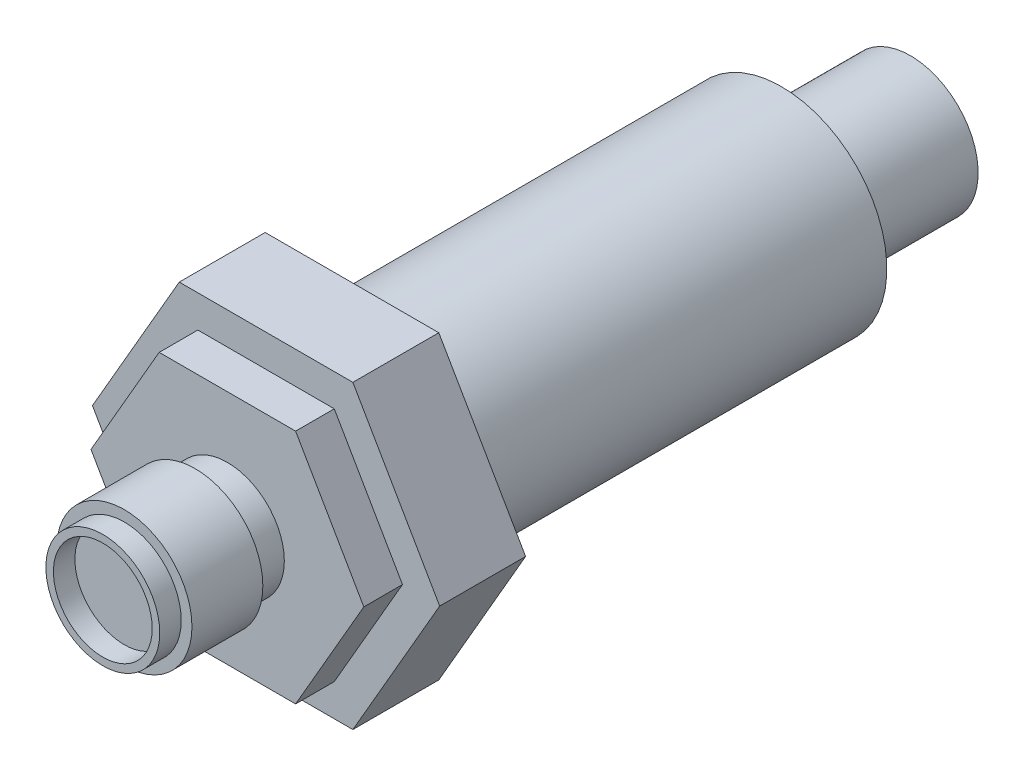
SolidWorks part; units mm, degrees
ref_plane "Front Plane" through (0, 0, 0) normal (0, 0, 1) x (1, 0, 0)
ref_plane "Top Plane" through (0, 0, 0) normal (0, 1, 0) x (1, 0, 0)
ref_plane "Right Plane" through (0, 0, 0) normal (1, 0, 0) x (0, 0, -1)
sketch "Sketch1" plane through (0, 0, 0) normal (0, 0, 1) x (1, 0, 0)
  line L1 (8.0829, 0) -> (4.0415, 7)
  line L2 (4.0415, 7) -> (-4.0415, 7)
  line L3 (-4.0415, 7) -> (-8.0829, 0)
  line L4 (-8.0829, 0) -> (-4.0415, -7)
  line L5 (-4.0415, -7) -> (4.0415, -7)
  line L6 (4.0415, -7) -> (8.0829, 0)
  circle A0 centre (0, 0) radius 7 construction
  dimension "D1" = 14
extrude "Boss-Extrude1" add sketch "Sketch1" along normal blind 4
sketch "Sketch2" plane through (0, 0, 4) normal (0, 0, 1) x (1, 0, 0)
  line L1 (6.3509, 0) -> (3.1754, 5.5)
  line L2 (3.1754, 5.5) -> (-3.1754, 5.5)
  line L3 (-3.1754, 5.5) -> (-6.3509, 0)
  line L4 (-6.3509, 0) -> (-3.1754, -5.5)
  line L5 (-3.1754, -5.5) -> (3.1754, -5.5)
  line L6 (3.1754, -5.5) -> (6.3509, 0)
  circle A0 centre (0, 0) radius 5.5 construction
  dimension "D1" = 11
extrude "Boss-Extrude2" add sketch "Sketch2" along normal blind 1.8
sketch "Sketch3" plane through (0, 0, 5.8) normal (0, 0, 1) x (1, 0, 0)
  circle A0 centre (0, 0) radius 2.65
  circle A1 centre (0, 0) radius 2.3
  dimension "D1" = 5.3
  dimension "D2" = 4.6
extrude "Boss-Extrude3" add sketch "Sketch3" along normal blind 5.8
sketch "Sketch4" plane through (0, 0, 11.6) normal (0, 0, 1) x (1, 0, 0)
  circle A0 centre (0, 0) radius 3.15
  dimension "D1" = 6.3
extrude "Boss-Extrude4" add sketch "Sketch4" against normal blind 3.3 from offset 1 offset against normal yes
cosmetic thread "Cosmetic Thread2" parameters "D2"=5.3
sketch "Sketch5" plane through (0, 0, 0) normal (0, 0, -1) x (-1, 0, 0)
  circle A0 centre (0, 0) radius 4.9
  dimension "D1" = 9.8
extrude "Boss-Extrude5" add sketch "Sketch5" along normal blind 20
cosmetic thread "Cosmetic Thread1" parameters "D2"=8.8
sketch "Sketch6" plane through (0, 0, -20) normal (0, 0, -1) x (-1, 0, 0)
  circle A0 centre (0, 0) radius 3.15
  circle A1 centre (0, 0) radius 2.25
  dimension "D1" = 6.3
  dimension "D2" = 4.5
extrude "Boss-Extrude6" add sketch "Sketch6" along normal blind 6
cosmetic thread "Cosmetic Thread3" parameters "D2"=5.3
